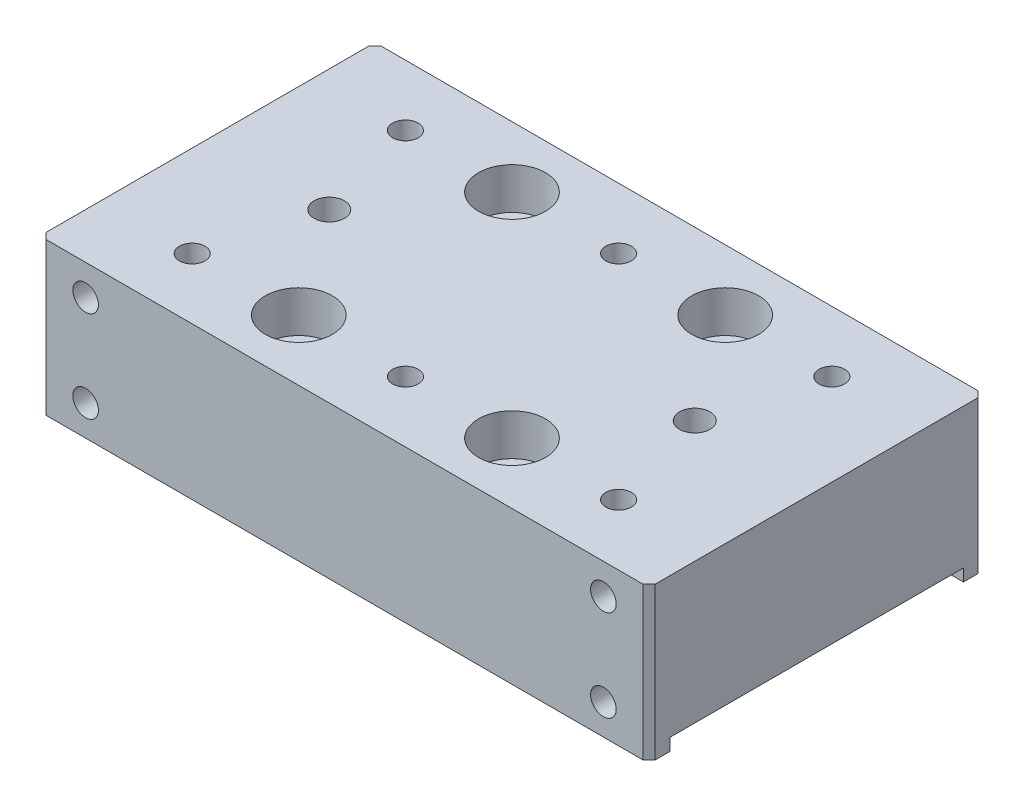
SolidWorks part; units mm, degrees
material "A6061 T6"
ref_plane "前视基准面" through (0, 0, 0) normal (0, 0, 1) x (1, 0, 0)
ref_plane "上视基准面" through (0, 0, 0) normal (0, 1, 0) x (1, 0, 0)
ref_plane "右视基准面" through (0, 0, 0) normal (1, 0, 0) x (0, 0, -1)
sketch "草图1" plane through (0, 0, 0) normal (0, 1, 0) x (1, 0, 0)
  line L1 (-50, 27.5) -> (50, 27.5)
  line L2 (-50, 27.5) -> (-50, -27.5)
  line L3 (-50, -27.5) -> (50, -27.5)
  line L4 (50, 27.5) -> (50, -27.5)
  line L5 (-50, 27.5) -> (50, -27.5) construction
  line L6 (-50, -27.5) -> (50, 27.5) construction
  point P0 (0, 0)
  dimension "D1" = 100
  dimension "D2" = 55
extrude "凸台-拉伸1" add sketch "草图1" along normal blind 25
sketch "草图2" plane through (50, 0, 0) normal (1, 0, 0) x (0, 0, -1)
  line L1 (-24.1, 2) -> (24.1, 2)
  line L2 (-24.1, 2) -> (-24.1, -2)
  line L3 (-24.1, -2) -> (24.1, -2)
  line L4 (24.1, 2) -> (24.1, -2)
  line L5 (-24.1, 2) -> (24.1, -2) construction
  line L6 (-24.1, -2) -> (24.1, 2) construction
  point P0 (0, 0)
  dimension "D1" = 48.2
  dimension "D2" = 4
extrude "切除-拉伸1" cut sketch "草图2" against normal through all
hole_wizard "M5 螺纹孔1" positions "草图3" profile "草图4" tap size "M5" standard "GB"
sketch "草图3" plane through (0, 0, 27.5) normal (0, 0, 1) x (1, 0, 0)
  line L0 (-50, 25) -> (50, 25) construction
  line L2 (-50, 25) -> (-50, 0) construction
  point P0 (42.5, 20)
  point P3 (42.5, 5)
  point P6 (-42.5, 20)
  point P8 (-42.5, 5)
  dimension "D1" = 5
  dimension "D2" = 15
  dimension "D3" = 7.5
sketch "草图4" plane through (42.5, 20, 27.5) normal (1, 0, 0) x (0, -1, 0)
  line L0 (0, 0) -> (0, 13.6618)
  line L1 (0, 13.6618) -> (2.1, 12.4)
  line L2 (2.1, 12.4) -> (2.1, 0)
  line L5 (2.1, 0) -> (0, 0)
  line L10 (0, 13.6618) -> (-2.1, 12.4) construction
  line L11 (0, -6.35) -> (0, 107.95) construction
  dimension "螺纹孔钻头直径" = 4.2
  dimension "螺纹孔钻头深度" = 12.4
  dimension "导头角度" = 118
cosmetic thread "孔螺蚊线9" parameters "D1"=10, "D2"=5
cosmetic thread "孔螺蚊线10" parameters "D1"=10, "D2"=5
cosmetic thread "孔螺蚊线11" parameters "D1"=10, "D2"=5
cosmetic thread "孔螺蚊线12" parameters "D1"=10, "D2"=5
chamfer "倒角1" distance 1 angle 45 4 edges at (-50, 12.5, -27.5) (-50, 12.5, 27.5) (50, 12.5, -27.5) (50, 12.5, 27.5)
hole_wizard "打孔尺寸(%根据)内六角圆柱头螺钉的类型0" positions "草图5" profile "草图6" counterbore size "M6" standard "GB"
sketch "草图5" plane through (0, 25, 0) normal (0, 1, 0) x (1, 0, 0)
  point P0 (-17.5, 17.5)
  point P3 (17.5, 17.5)
  point P6 (-17.5, -17.5)
  point P9 (17.5, -17.5)
sketch "草图6" plane through (-17.5, 25, -17.5) normal (1, 0, 0) x (0, 0, 1)
  line L0 (0, 0) -> (0, 41.9828)
  line L1 (0, 41.9828) -> (3.3, 40)
  line L2 (3.3, 40) -> (3.3, 6.8)
  line L3 (3.3, 6.8) -> (5.5, 6.8)
  line L4 (5.5, 6.8) -> (5.5, 0)
  line L5 (5.5, 0) -> (0, 0)
  line L10 (0, 41.9828) -> (-3.3, 40) construction
  line L11 (0, -6.35) -> (0, 107.95) construction
  dimension "孔直径" = 6.6
  dimension "孔深度" = 40
  dimension "柱形沉头孔直径" = 11
  dimension "柱形沉头孔深度" = 6.8
  dimension "导头角度" = 118
hole_wizard "M5 螺纹孔2" positions "草图7" profile "草图8" tap size "M5" standard "GB"
sketch "草图7" plane through (0, 25, 0) normal (0, 1, 0) x (1, 0, 0)
  line L0 (-50, 26.5) -> (-50, -26.5) construction
  line L1 (50, -26.5) -> (50, 26.5) construction
  line L2 (49, 27.5) -> (-49, 27.5) construction
  line L3 (-49, -27.5) -> (49, -27.5) construction
  point P0 (-35, 17.5)
  point P2 (-35, -17.5)
  point P4 (35, 17.5)
  point P6 (35, -17.5)
  point P9 (0, 17.5)
  point P11 (0, -17.5)
  dimension "D1" = 15
  dimension "D2" = 15
  dimension "D3" = 10
  dimension "D4" = 10
  dimension "D5" = 35
sketch "草图8" plane through (-35, 25, -17.5) normal (1, 0, 0) x (0, 0, 1)
  line L0 (0, 0) -> (0, 13.6618)
  line L1 (0, 13.6618) -> (2.1, 12.4)
  line L2 (2.1, 12.4) -> (2.1, 0)
  line L5 (2.1, 0) -> (0, 0)
  line L10 (0, 13.6618) -> (-2.1, 12.4) construction
  line L11 (0, -6.35) -> (0, 107.95) construction
  dimension "螺纹孔钻头直径" = 4.2
  dimension "螺纹孔钻头深度" = 12.4
  dimension "导头角度" = 118
cosmetic thread "孔螺蚊线3" parameters "D1"=10, "D2"=5
cosmetic thread "孔螺蚊线4" parameters "D1"=10, "D2"=5
cosmetic thread "孔螺蚊线5" parameters "D1"=10, "D2"=5
cosmetic thread "孔螺蚊线6" parameters "D1"=10, "D2"=5
cosmetic thread "孔螺蚊线7" parameters "D1"=10, "D2"=5
cosmetic thread "孔螺蚊线8" parameters "D1"=10, "D2"=5
hole_wizard "大小mm 暗销孔1" positions "草图9" profile "草图10" hole size "Ø5.0" standard "GB"
sketch "草图9" plane through (0, 25, 0) normal (0, 1, 0) x (1, 0, 0)
  line L0 (-50, 26.5) -> (-50, -26.5) construction
  line L1 (50, -26.5) -> (50, 26.5) construction
  line L2 (49, 27.5) -> (-49, 27.5) construction
  point P0 (-30, 0)
  point P2 (30, 0)
  dimension "D1" = 20
  dimension "D2" = 20
  dimension "D3" = 27.5
sketch "草图10" plane through (-30, 25, 0) normal (1, 0, 0) x (0, 0, 1)
  line L0 (0, 0) -> (0, 13.9022)
  line L1 (0, 13.9022) -> (2.5, 12.4)
  line L2 (2.5, 12.4) -> (2.5, 0)
  line L5 (2.5, 0) -> (0, 0)
  line L10 (0, 13.9022) -> (-2.5, 12.4) construction
  line L11 (0, -6.35) -> (0, 107.95) construction
  dimension "孔直径" = 5
  dimension "孔深度" = 12.4
  dimension "导头角度" = 118
